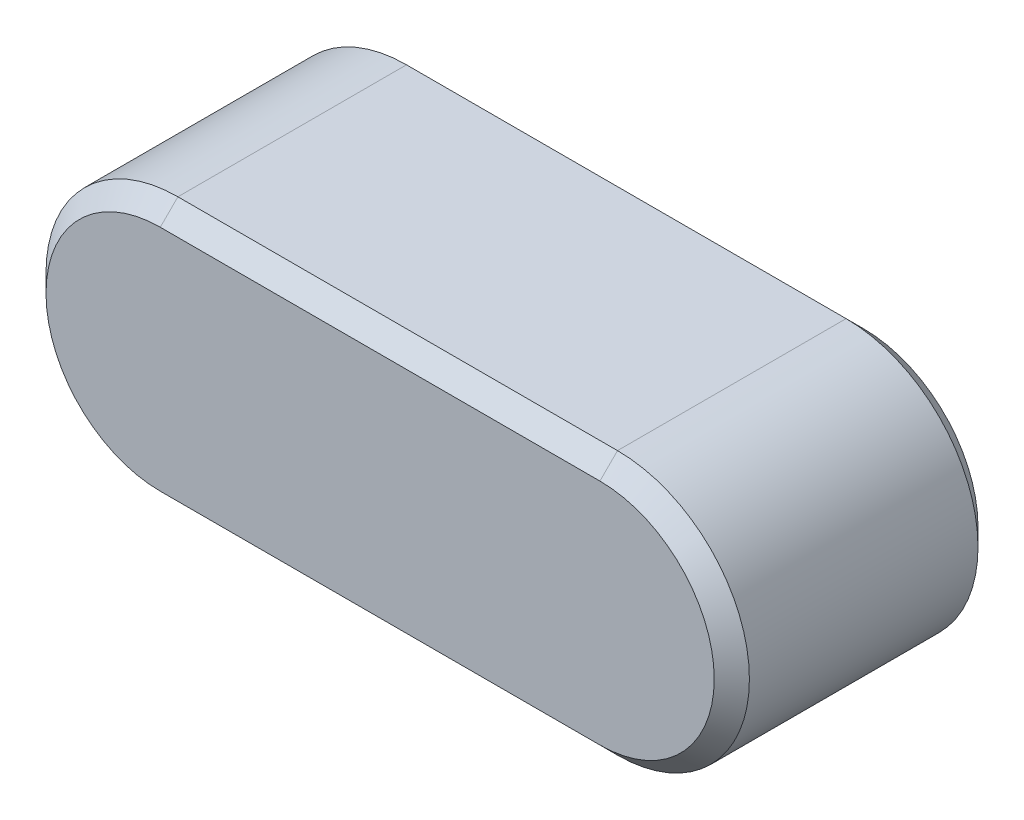
from build123d import *

# Parameters (mm, degrees)
BASEKEY_DEPTH = 3
CHAMFER1_SIZE = 0.4


with BuildPart() as part:
    # Sketch1 → BaseKey (new, symmetric)
    with BuildSketch(Plane.XY):
        with BuildLine():
            Line((-10, 3), (0, 3))
            ThreePointArc((0, 3), (3, 0), (0, -3))
            Line((0, -3), (-10, -3))
            ThreePointArc((-10, -3), (-13, 0), (-10, 3))
        make_face()
    extrude(amount=BASEKEY_DEPTH, both=True)

    # Chamfer1
    chamfer1_edges = [part.edges().sort_by_distance(p)[0] for p in [
        (3, 0, 3),
        (-5, 3, 3),
        (-13, 0, 3),
        (-5, 3, -3),
        (3, 0, -3),
        (-5, -3, -3),
        (-13, 0, -3),
        (-5, -3, 3),
    ]]
    chamfer(chamfer1_edges, length=CHAMFER1_SIZE)


solid = part.part
